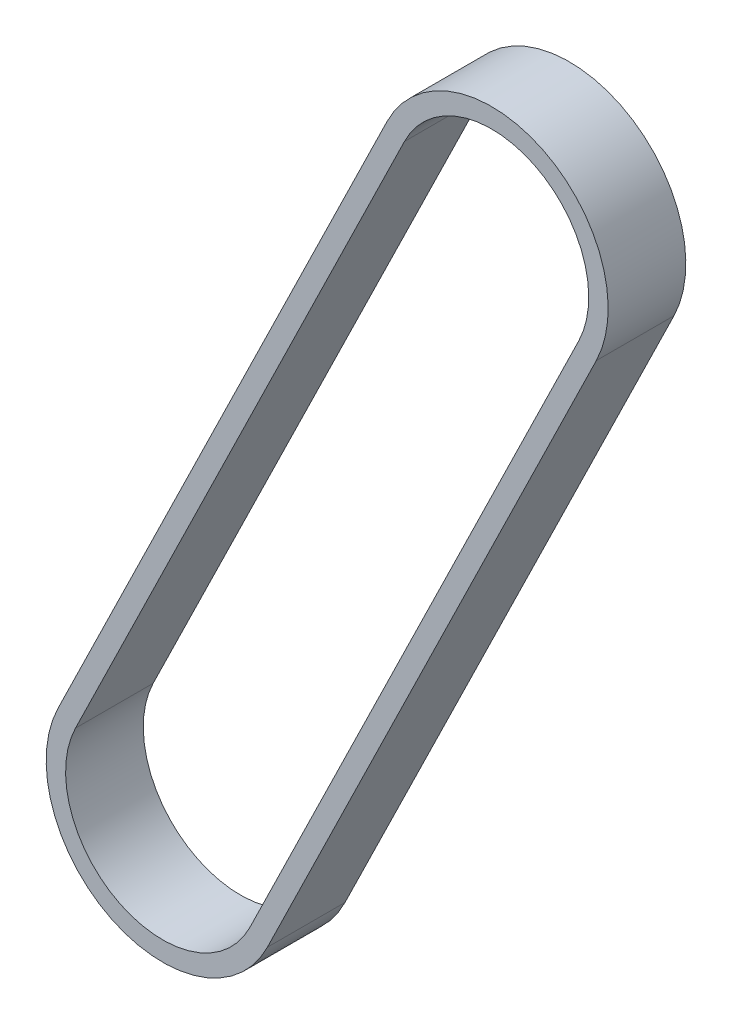
SolidWorks part; units mm, degrees
ref_plane "前视基准面" through (0, 0, 0) normal (0, 0, 1) x (1, 0, 0)
ref_plane "上视基准面" through (0, 0, 0) normal (0, 1, 0) x (1, 0, 0)
ref_plane "右视基准面" through (0, 0, 0) normal (1, 0, 0) x (0, 0, -1)
other "Configuration Table"
sketch "草图1" plane through (0, 0, 0) normal (0, 0, 1) x (1, 0, 0)
  line L0 (896.6188, 885.7376) -> (557.7612, 192.9556)
  line L1 (1076.2789, 797.8612) -> (737.4213, 105.0792)
  line L2 (878.6528, 894.5252) -> (539.7952, 201.7432)
  line L3 (1094.2449, 789.0735) -> (755.3873, 96.2916)
  arc A1 (1076.2789, 797.8612) -> (896.6188, 885.7376) centre (986.4488, 841.7994) ccw
  arc A3 (557.7612, 192.9556) -> (737.4213, 105.0792) centre (647.5913, 149.0174) ccw
  arc A4 (539.7952, 201.7432) -> (755.3873, 96.2916) centre (647.5913, 149.0174) ccw
  arc A5 (1094.2449, 789.0735) -> (878.6528, 894.5252) centre (986.4488, 841.7994) ccw
  dimension "D1" = 20
extrude "凸台-拉伸1" add sketch "草图1" along normal mid plane 80
